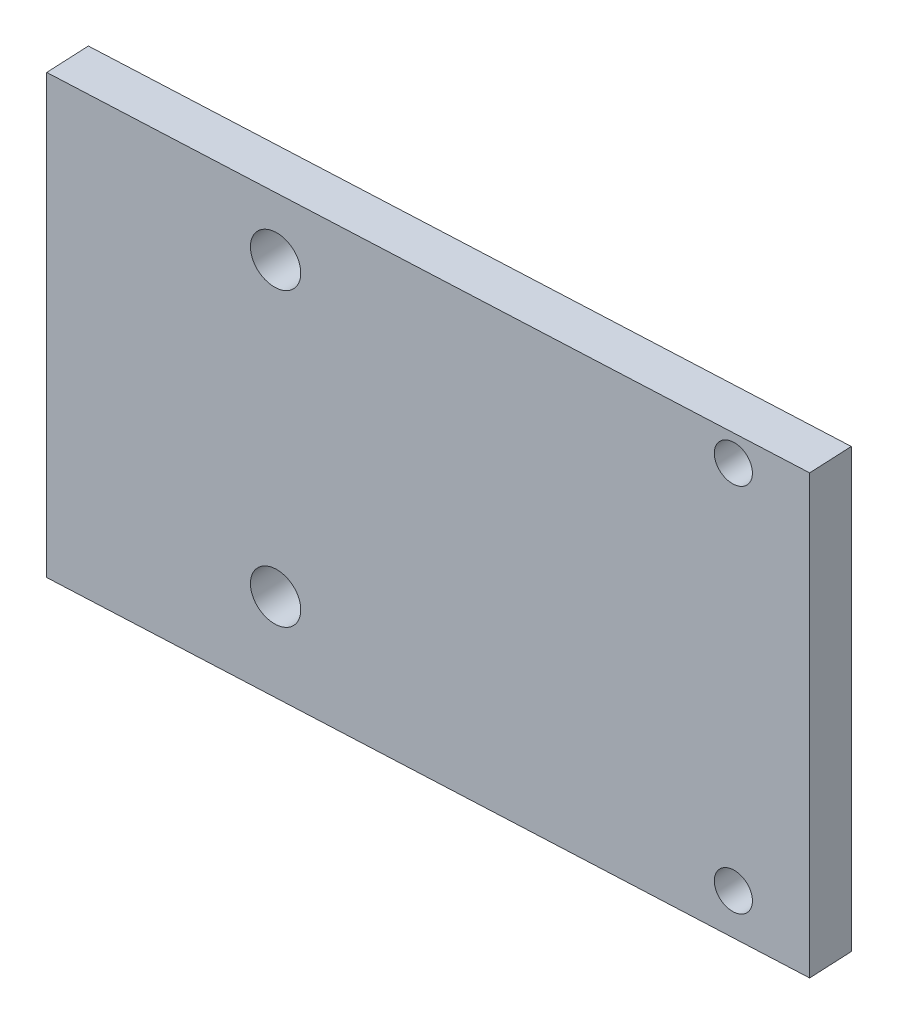
from build123d import *

# Parameters (mm, degrees)
SKETCH1_W           = 50
SKETCH1_H           = 30
BOSS_EXTRUDE1_DEPTH = 3
M4_TAPPED_HOLE1_D   = 3.3
M3_TAPPED_HOLE1_D   = 2.5


with BuildPart() as part:
    # Sketch1 → Boss-Extrude1 (new body)
    with BuildSketch(Plane(origin=(18.523271638, 0, -0.440780543), x_dir=(-0.9988681377244376, 0, 0.04756514941544916), z_dir=(-0.04756514941544916, 0, -0.9988681377244377))):
        with Locations((7.591880235, 309)):
            Rectangle(SKETCH1_W, SKETCH1_H)
    extrude(amount=-BOSS_EXTRUDE1_DEPTH)

    # M4 Tapped Hole1 (through all)
    with Locations(Plane(origin=(0.020965792, 0, 0.44028164), x_dir=(-0.9988681377244376, 0, 0.04756514941544917), z_dir=(-0.047565149415449176, 0, -0.9988681377244377))):
        with Locations((-0.931391403, 320), (-0.931391403, 300)):
            Hole(M4_TAPPED_HOLE1_D / 2)

    # M3 Tapped Hole1 (through all)
    with Locations(Plane(origin=(0.020965792, 0, 0.44028164), x_dir=(-0.9988681377244376, 0, 0.04756514941544917), z_dir=(-0.047565149415449176, 0, -0.9988681377244377))):
        with Locations((-30.931391403, 322.2), (-30.931391403, 296.8)):
            Hole(M3_TAPPED_HOLE1_D / 2)


solid = part.part
